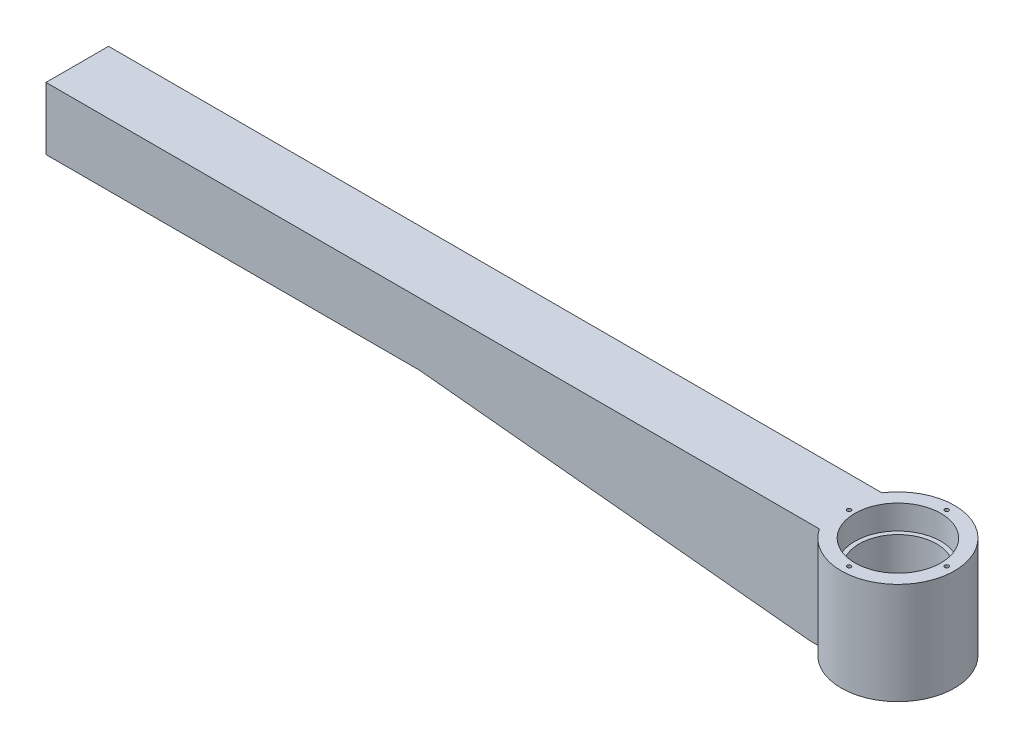
SolidWorks part; units mm, degrees
ref_plane "Front Plane" through (0, 0, 0) normal (0, 0, 1) x (1, 0, 0)
ref_plane "Top Plane" through (0, 0, 0) normal (0, 1, 0) x (1, 0, 0)
ref_plane "Right Plane" through (0, 0, 0) normal (1, 0, 0) x (0, 0, -1)
sketch "Sketch1" plane through (0, 0, 0) normal (0, 0, 1) x (1, 0, 0)
  line L0 (0, 0) -> (0, 133.461) construction
  line L1 (-55, 0) -> (-72.5, 0)
  line L2 (-72.5, 0) -> (-72.5, 130)
  line L3 (-72.5, 130) -> (-55, 130)
  line L4 (-55, 130) -> (-55, 99)
  line L5 (-55, 99) -> (-49.5, 99)
  line L6 (-49.5, 99) -> (-49.5, 31)
  line L7 (-49.5, 31) -> (-55, 31)
  line L8 (-55, 31) -> (-55, 0)
  dimension "D1" = 130
  dimension "D2" = 72.5
  dimension "D3" = 49.5
  dimension "D4" = 55
  dimension "D5" = 31
  dimension "D6" = 31
revolve "Revolve1" add sketch "Sketch1" angle 360 about L0
hole_wizard "M6 Tapped Hole1" positions "Sketch3" profile "Sketch2" tap size "M6" standard "Gb"
sketch "Sketch3" plane through (0, 130, 0) normal (0, 1, 0) x (1, 0, 0)
  point P0 (0, 62.5)
  dimension "D1" = 62.5
sketch "Sketch2" plane through (0, 130, -62.5) normal (1, 0, 0) x (0, 0, 1)
  line L0 (0, 0) -> (0, 19.5022)
  line L1 (0, 19.5022) -> (2.5, 18)
  line L2 (2.5, 18) -> (2.5, 0)
  line L5 (2.5, 0) -> (0, 0)
  line L10 (0, 19.5022) -> (-2.5, 18) construction
  line L11 (0, -6.35) -> (0, 107.95) construction
  dimension "螺纹孔钻头直径" = 5
  dimension "螺纹孔钻头深度" = 18
  dimension "导头角度" = 118
cosmetic thread "Cosmetic thread1" parameters "D1"=15, "D2"=6
pattern_circular "CirPattern1" count 4 over 360 about axis through (0, 0, 0) along (0, 1, 0) of "M6 Tapped Hole1"
hole_wizard "M6 Tapped Hole2" positions "Sketch5" profile "Sketch4" tap size "M6" standard "Gb"
sketch "Sketch5" plane through (0, 0, 0) normal (0, -1, 0) x (-1, 0, 0)
  point P0 (0, -62.5)
  dimension "D1" = 62.5
sketch "Sketch4" plane through (0, 0, 62.5) normal (1, 0, 0) x (0, 0, -1)
  line L0 (0, 0) -> (0, 19.5022)
  line L1 (0, 19.5022) -> (2.5, 18)
  line L2 (2.5, 18) -> (2.5, 0)
  line L5 (2.5, 0) -> (0, 0)
  line L10 (0, 19.5022) -> (-2.5, 18) construction
  line L11 (0, -6.35) -> (0, 107.95) construction
  dimension "螺纹孔钻头直径" = 5
  dimension "螺纹孔钻头深度" = 18
  dimension "导头角度" = 118
cosmetic thread "Cosmetic thread2" parameters "D1"=15, "D2"=6
pattern_circular "CirPattern2" count 4 over 360 about axis through (0, 0, 0) along (0, 1, 0) of "M6 Tapped Hole2"
sketch "Sketch6" plane through (0, 130, 0) normal (0, 1, 0) x (1, 0, 0)
  line L0 (-1050, 40) -> (-60.4669, 40)
  line L1 (-1050, -40) -> (-60.4669, -40)
  line L2 (-1050, -40) -> (-1050, 40)
  circle A0 centre (0, 0) radius 72.5 construction
  arc A1 (-60.4669, 40) -> (-60.4669, -40) centre (0, 0) ccw
  dimension "D1" = 1050
  dimension "D2" = 80
  dimension "D3" = 40
extrude "Boss-Extrude1" add sketch "Sketch6" against normal blind 80 separate body
shell "Shell1" thickness 6
sketch "Sketch8" plane through (0, 0, 40) normal (0, 0, 1) x (1, 0, 0)
  line L0 (-60.4669, 50) -> (-572.5, 50)
  line L1 (-60.4669, 50) -> (-60.4669, 130) construction
  line L2 (-1050, 50) -> (-60.4669, 50) construction
  line L3 (-572.5, 50) -> (-72.5, 0)
  line L4 (-72.5, 130) -> (-72.5, 0) construction
  line L5 (-72.5, 0) -> (-60.4669, 0)
  line L6 (-72.5, 0) -> (72.5, 0) construction
  line L7 (-60.4669, 0) -> (-60.4669, 50)
  dimension "D1" = 500
extrude "Boss-Extrude3" add sketch "Sketch8" against normal blind 6
mirror "Mirror1" about plane through (0, 0, 0) normal (0, 0, 1) of "Boss-Extrude3"
